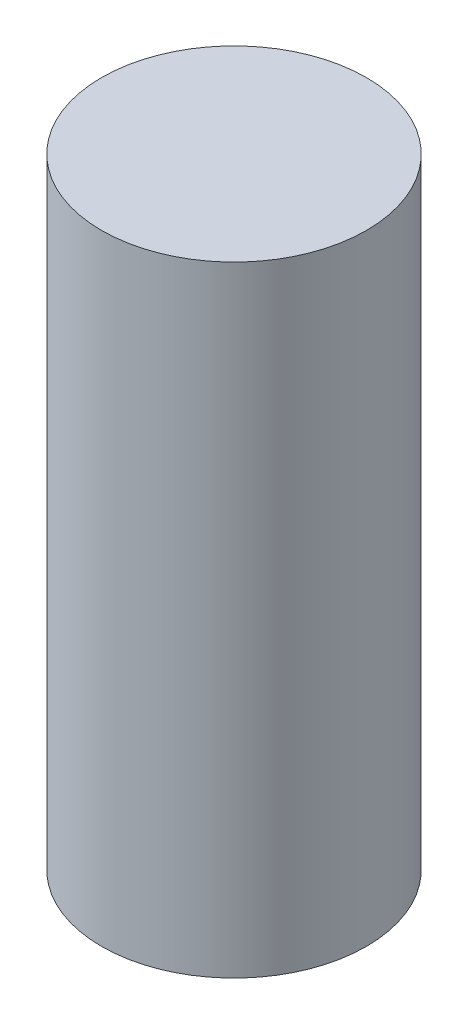
from build123d import *

# Parameters (mm, degrees)
SKETCH1_R           = 35
BOSS_EXTRUDE1_DEPTH = 163.9


with BuildPart() as part:
    # Sketch1 → Boss-Extrude1 (new body)
    with BuildSketch(Plane(origin=(0, 0, 0), x_dir=(1, 0, 0), z_dir=(0, 1, 0))):
        with Locations(Location((0, 0, 0), (0, 0, 270))):
            Circle(SKETCH1_R)
    extrude(amount=BOSS_EXTRUDE1_DEPTH)


solid = part.part
